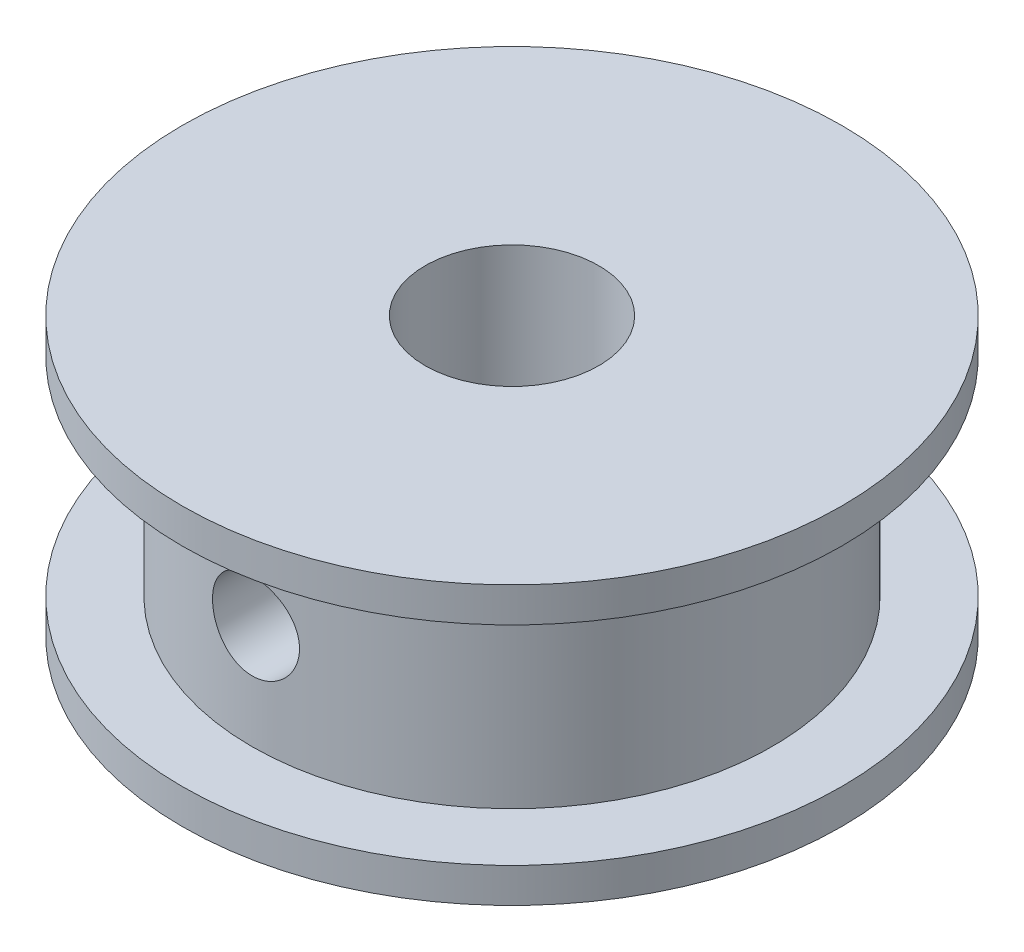
SolidWorks part; units mm, degrees
ref_plane "前视基准面" through (0, 0, 0) normal (0, 0, 1) x (1, 0, 0)
ref_plane "上视基准面" through (0, 0, 0) normal (0, 1, 0) x (1, 0, 0)
ref_plane "右视基准面" through (0, 0, 0) normal (1, 0, 0) x (0, 0, -1)
sketch "草图1" plane through (0, 0, 0) normal (0, 0, 1) x (1, 0, 0)
  line L0 (0, 18.9135) -> (0, -19.303) construction
  line L1 (9.5, 9.117) -> (2.5, 9.117)
  line L2 (9.5, 9.117) -> (9.5, 8.117)
  line L3 (9.5, 8.117) -> (7.5, 8.117)
  line L4 (7.5, 8.117) -> (7.5, 2.117)
  line L5 (7.5, 2.117) -> (9.5, 2.117)
  line L6 (9.5, 2.117) -> (9.5, 1.117)
  line L7 (9.5, 1.117) -> (2.5, 1.117)
  line L8 (2.5, 9.117) -> (2.5, 1.117)
  dimension "D1" = 2.5
  dimension "D2" = 9.5
  dimension "D3" = 9.5
  dimension "D4" = 8
  dimension "D5" = 1
  dimension "D6" = 1
  dimension "D7" = 7.5
revolve "旋转1" add sketch "草图1" angle 360 about L0
hole_wizard "M3 螺纹孔1" positions "3D草图6" profile "草图9" tap size "M3" standard "Iso"
sketch3d "3D草图6"
  point P0 (0.0195, 5.1355, 7.5)
sketch "草图9" plane through (0.0195, 5.1355, 7.5) normal (0, 1, 0) x (1, 0, -0.0026)
  line L0 (0, 0) -> (0, 5)
  line L1 (0, 5) -> (1.25, 5)
  line L2 (1.25, 5) -> (1.25, 0)
  line L5 (1.25, 0) -> (0, 0)
  line L11 (0, -6.35) -> (0, 107.95) construction
  dimension "通孔螺纹孔钻头直径" = 2.5
  dimension "通孔螺纹孔钻头深度" = 5
cosmetic thread "孔螺蚊线1" parameters "D2"=3
